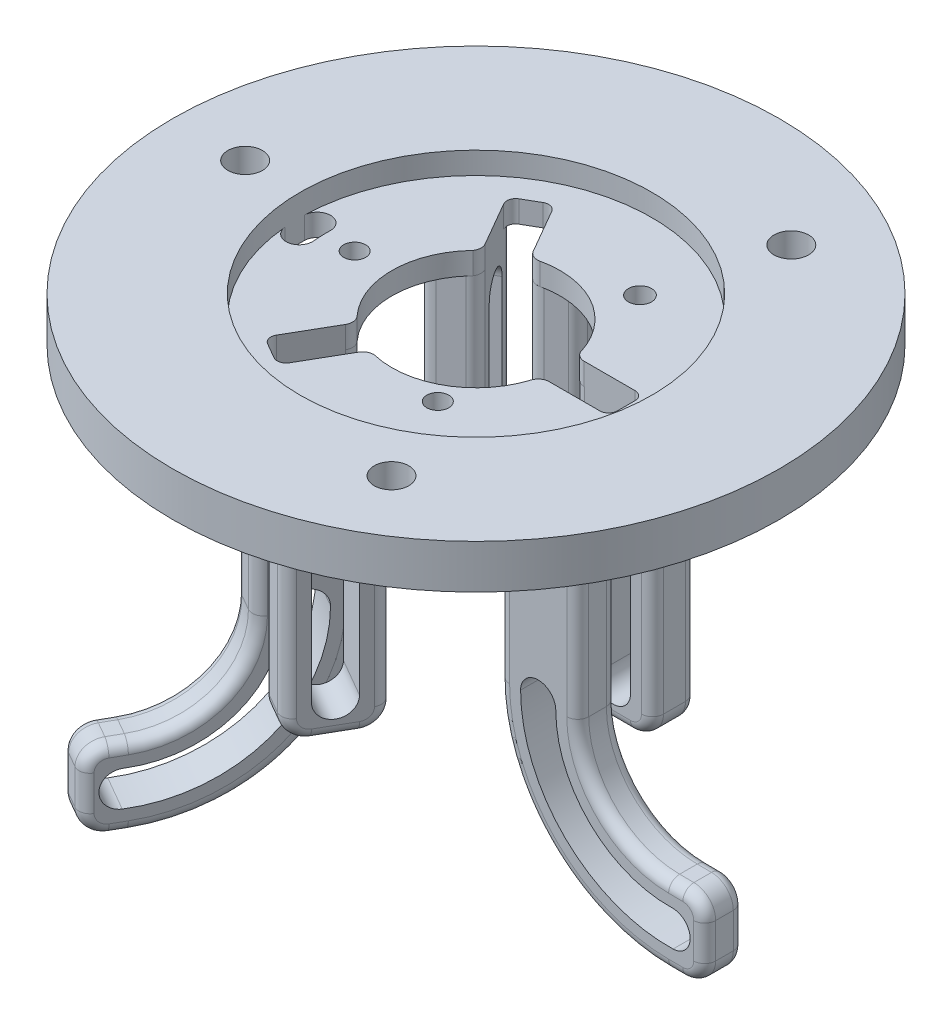
from build123d import *

# Parameters (mm, degrees)
SKETCH1_R           = 138
BOSS_EXTRUDE1_DEPTH = 20
BOSS_EXTRUDE2_START = 8
BOSS_EXTRUDE2_DEPTH = 18
CUT_EXTRUDE5_DEPTH  = 34
BOSS_EXTRUDE3_START = -70
SKETCH7_W           = 46
SKETCH7_H           = 125.96740774
BOSS_EXTRUDE3_DEPTH = 20
CUT_EXTRUDE6_START  = -72
CUT_EXTRUDE6_DEPTH  = 45
CUT_EXTRUDE7_DEPTH  = 72
CIRPATTERN1_COUNT   = 3
CUT_EXTRUDE8_DEPTH  = 27
CUT_EXTRUDE10_DEPTH = 27
CIRPATTERN4_COUNT   = 3
CIRPATTERN5_COUNT   = 3
FILLET2_R           = 10
SKETCH12_R          = 7.875
CUT_EXTRUDE11_DEPTH = 27
CIRPATTERN8_COUNT   = 3
FILLET3_R           = 5
CUT_EXTRUDE12_DEPTH = 27
CUT_EXTRUDE13_DEPTH = 27
SKETCH17_R          = 80
CUT_EXTRUDE14_DEPTH = 10
CUT_EXTRUDE15_DEPTH = 10
SKETCH19_R          = 5
SKETCH19_R_2        = 5.269356663
CUT_EXTRUDE16_DEPTH = 10


with BuildPart() as part:
    # Sketch1 → Boss-Extrude1 (new body)
    with BuildSketch(Plane(origin=(0, 0, 0), x_dir=(1, 0, 0), z_dir=(0, 1, 0))):
        with Locations(Location((0, 0, 0), (0, 0, 270))):
            Circle(SKETCH1_R)
    extrude(amount=BOSS_EXTRUDE1_DEPTH)

    # Sketch2 → Boss-Extrude2 (add)
    with BuildSketch(Plane.XY.offset(BOSS_EXTRUDE2_START)):
        Polygon((36.291327226, 0), (36.291327226, -145.182091657), (89.27461892, -189.63281459), (138, -189.63281459), (138, -149.439703236), (82.291327226, -93.731030462), (82.291327226, 0), align=None)
    boss_extrude2 = extrude(amount=BOSS_EXTRUDE2_DEPTH)

    # Sketch4 → Cut-Extrude5 (cut)
    with BuildSketch(Plane.XY.offset(8)):
        with BuildLine():
            ThreePointArc((46.291327226, -100), (66.736553538, -148.33011915), (115.658506664, -167.315645172))
            ThreePointArc((115.658506664, -167.315645172), (123.414805799, -159.07915176), (115.178312386, -151.322852625))
            ThreePointArc((115.178312386, -151.322852625), (77.879194418, -136.847891395), (62.291327226, -100))
            ThreePointArc((62.291327226, -100), (54.291327226, -92), (46.291327226, -100))
        make_face()
    cut_extrude5 = extrude(amount=CUT_EXTRUDE5_DEPTH, mode=Mode.SUBTRACT)

    # Sketch7 → Boss-Extrude3 (add)
    with BuildSketch(Plane.XY.offset(42).offset(BOSS_EXTRUDE3_START)):
        with Locations((59.291327226, -62.98370387)):
            Rectangle(SKETCH7_W, SKETCH7_H)
    boss_extrude3 = extrude(amount=BOSS_EXTRUDE3_DEPTH)

    # Sketch3 → Cut-Extrude6 (cut)
    with BuildSketch(Plane.XY.offset(26).offset(CUT_EXTRUDE6_START)):
        with BuildLine():
            Line((46.291327226, -17.246577518), (46.291327226, -110.518557102))
            ThreePointArc((46.291327226, -110.518557102), (54.291327226, -118.518557102), (62.291327226, -110.518557102))
            Line((62.291327226, -110.518557102), (62.291327226, -17.246577518))
            ThreePointArc((62.291327226, -17.246577518), (54.291327226, -9.246577518), (46.291327226, -17.246577518))
        make_face()
    cut_extrude6 = extrude(amount=CUT_EXTRUDE6_DEPTH, mode=Mode.SUBTRACT)

    # Sketch8 → Cut-Extrude7 (cut)
    with BuildSketch(Plane.XY.offset(26)):
        Polygon((138, -149.439703236), (130.041059052, -141.480762288), (130.041059052, -169.782953928), (130.057177794, -189.63281459), (138, -189.63281459), align=None)
    cut_extrude7 = extrude(amount=-CUT_EXTRUDE7_DEPTH, mode=Mode.SUBTRACT)

    # CirPattern1: Boss-Extrude2, Cut-Extrude5, Boss-Extrude3, Cut-Extrude6, Cut-Extrude7 ×3 about axis
    cirpattern1_axis = Axis((0, 0, 0), (0, 1, 0))
    add([boss_extrude2.rotate(cirpattern1_axis, i * 360 / CIRPATTERN1_COUNT) for i in range(1, CIRPATTERN1_COUNT)])
    add([cut_extrude5.rotate(cirpattern1_axis, i * 360 / CIRPATTERN1_COUNT) for i in range(1, CIRPATTERN1_COUNT)], mode=Mode.SUBTRACT)
    add([boss_extrude3.rotate(cirpattern1_axis, i * 360 / CIRPATTERN1_COUNT) for i in range(1, CIRPATTERN1_COUNT)])
    add([cut_extrude6.rotate(cirpattern1_axis, i * 360 / CIRPATTERN1_COUNT) for i in range(1, CIRPATTERN1_COUNT)], mode=Mode.SUBTRACT)
    add([cut_extrude7.rotate(cirpattern1_axis, i * 360 / CIRPATTERN1_COUNT) for i in range(1, CIRPATTERN1_COUNT)], mode=Mode.SUBTRACT)

    # Sketch9 → Cut-Extrude8 (cut)
    with BuildSketch(Plane(origin=(0, 0, -28), x_dir=(-1, 0, 0), z_dir=(0, 0, -1))):
        Polygon((-72.291327226, -43.273748779), (-72.291327226, 0), (-82.291327226, 0), (-82.291327226, -125.96740774), (-72.291327226, -125.96740774), align=None)
    cut_extrude8 = extrude(amount=-CUT_EXTRUDE8_DEPTH, mode=Mode.SUBTRACT)

    # Sketch11 → Cut-Extrude10 (cut)
    with BuildSketch(Plane.XY.offset(26)):
        with BuildLine():
            Line((36.291327226, -100), (36.291327226, -145.182091657))
            Line((36.291327226, -145.182091657), (89.27461892, -189.63281459))
            Line((89.27461892, -189.63281459), (130.057177794, -189.63281459))
            Line((130.057177794, -189.63281459), (134.49428622, -177.345982234))
            Line((134.49428622, -177.345982234), (113.63730946, -177.345982234))
            ThreePointArc((113.63730946, -177.345982234), (58.945440925, -154.691868535), (36.291327226, -100))
        make_face()
        with BuildLine():
            Line((72.28730946, -100), (72.28730946, 0))
            Line((72.28730946, 0), (138, 0))
            Line((138, 0), (154.98730946, -100))
            ThreePointArc((154.98730946, -100), (151.644308961, -116.287740448), (142.155846877, -129.941869073))
            Line((142.155846877, -129.941869073), (130.041059052, -141.480762288))
            Line((130.041059052, -141.480762288), (113.63730946, -141.35))
            ThreePointArc((113.63730946, -141.35), (84.398444058, -129.238865402), (72.28730946, -100))
        make_face()
    cut_extrude10 = extrude(amount=-CUT_EXTRUDE10_DEPTH, mode=Mode.SUBTRACT)

    # CirPattern4: Cut-Extrude8 ×3 about axis
    cirpattern4_axis = Axis((0, 20, 0), (0, -1, 0))
    for i in range(1, CIRPATTERN4_COUNT):
        add(cut_extrude8.rotate(cirpattern4_axis, i * 360 / CIRPATTERN4_COUNT), mode=Mode.SUBTRACT)

    # CirPattern5: Cut-Extrude10 ×3 about axis
    cirpattern5_axis = Axis((0, 0, 0), (0, 1, 0))
    for i in range(1, CIRPATTERN5_COUNT):
        add(cut_extrude10.rotate(cirpattern5_axis, i * 360 / CIRPATTERN5_COUNT), mode=Mode.SUBTRACT)

    # Fillet2
    fillet2_edges = [part.edges().sort_by_distance(p)[0] for p in [
        (-2.557206345, -125.96740774, 40.429211315),
        (-33.734120881, -125.96740774, -22.429211315),
        (-79.74296139, -141.480762288, 104.118860674),
        (-50.298097662, -141.480762288, -121.118860674),
        (72.291327226, -125.96740774, -18),
        (130.04720048, -177.345982234, 17),
        (-51.734120881, -125.96740774, -53.606125851),
        (-20.557206345, -125.96740774, 71.606125851),
        (-79.746032105, -177.345982234, 104.124179307),
        (-50.301168376, -177.345982234, -121.124179307),
        (36.291327226, -125.96740774, -18),
        (130.041059052, -141.480762288, 17),
    ]]
    fillet(fillet2_edges, radius=FILLET2_R)

    # Sketch12 → Cut-Extrude11 (cut)
    with BuildSketch(Plane(origin=(0, 20, 0), x_dir=(1, 0, 0), z_dir=(0, 1, 0))):
        with Locations(Location((-105, 0, 0), (0, 0, 270))):
            Circle(SKETCH12_R)
    cut_extrude11 = extrude(amount=-CUT_EXTRUDE11_DEPTH, mode=Mode.SUBTRACT)

    # CirPattern8: Cut-Extrude11 ×3 about axis
    cirpattern8_axis = Axis((0, 0, 0), (0, 1, 0))
    for i in range(1, CIRPATTERN8_COUNT):
        add(cut_extrude11.rotate(cirpattern8_axis, i * 360 / CIRPATTERN8_COUNT), mode=Mode.SUBTRACT)

    # Fillet3
    fillet3_edges = [part.edges().sort_by_distance(p)[0] for p in [
        (-25.073866843, -50, 27.429211315),
        (36.291327226, -50, 26),
        (-40.662324111, -50, 18.429211315),
        (-11.217460383, -50, -35.429211315),
        (4.370996885, -50, -44.429211315),
        (6.103047693, -57.98370387, 45.429211315),
        (-11.217460383, -57.98370387, 35.429211315),
        (-42.394374919, -57.98370387, -17.429211315),
        (-25.073866843, -57.98370387, -27.429211315),
        (72.291327226, -57.98370387, -8),
        (58.945440925, -154.691868535, 8),
        (58.945440925, -154.691868535, 26),
        (72.28730946, -50, 26),
        (84.398444058, -129.238865402, 26),
        (116.879040428, -141.375841419, 26),
        (84.398444058, -129.238865402, 8),
        (72.28730946, -50, 8),
        (116.879040428, -141.375841419, 8),
        (-43.073866843, -57.98370387, -58.606125851),
        (-29.217460383, -57.98370387, 66.606125851),
        (-22.544517232, -154.691868535, -55.048249278),
        (-6.956059964, -154.691868535, -64.048249278),
        (-58.660315228, -50, 49.602646364),
        (-64.715882527, -129.238865402, 60.091196594),
        (-80.956180712, -141.375841419, 88.220218181),
        (-49.127425259, -129.238865402, 69.091196594),
        (-43.07185796, -50, 58.602646364),
        (-65.367723444, -141.375841419, 97.220218181),
        (-36.400923693, -154.691868535, 47.048249278),
        (-51.989380961, -154.691868535, 38.048249278),
        (36.291327226, -57.98370387, -28),
        (-13.626994232, -50, -75.602646364),
        (-19.682561531, -129.238865402, -86.091196594),
        (-35.922859716, -141.375841419, -114.220218181),
        (-35.271018799, -129.238865402, -77.091196594),
        (-29.2154515, -50, -66.602646364),
        (-51.511316984, -141.375841419, -105.220218181),
        (36.291327226, -57.98370387, -8),
        (-42.503869028, -159.373673682, -125.618860674),
        (-58.092326296, -159.373673682, -116.618860674),
        (-35.90293163, -177.345982234, -114.185701723),
        (-41.039402933, -174.417050046, -123.082330993),
        (-41.053466248, -144.358536274, -123.106689369),
        (-51.491388898, -177.345982234, -105.185701723),
        (-56.627860202, -174.417050046, -114.082330993),
        (-56.641923516, -144.358536274, -114.106689369),
        (-87.537190024, -159.373673682, 99.618860674),
        (-71.948732756, -159.373673682, 108.618860674),
        (-80.936252626, -177.345982234, 88.185701723),
        (-86.07272393, -174.417050046, 97.082330993),
        (-86.086787245, -144.358536274, 97.106689369),
        (-65.347795358, -177.345982234, 97.185701723),
        (-70.484266662, -174.417050046, 106.082330993),
        (-70.498329977, -144.358536274, 106.106689369),
        (-60.394374919, -57.98370387, -48.606125851),
        (-51.394374919, -125.96740774, -33.017668583),
        (-43.858841013, -123.038475552, -19.965740996),
        (-58.929908825, -123.038475552, -46.06959617),
        (-34.073866843, -125.96740774, -43.017668583),
        (-26.538332937, -123.038475552, -29.965740996),
        (-41.609400749, -123.038475552, -56.06959617),
        (-2.896952307, -125.96740774, 61.017668583),
        (-20.217460383, -125.96740774, 51.017668583),
        (-11.896952307, -57.98370387, 76.606125851),
        (-10.432486213, -123.038475552, 74.06959617),
        (4.638581599, -123.038475552, 47.965740996),
        (-27.752994289, -123.038475552, 64.06959617),
        (-12.681926477, -123.038475552, 37.965740996),
        (54.291327226, -125.96740774, -28),
        (54.291327226, -125.96740774, -8),
        (72.291327226, -57.98370387, -28),
        (69.362395038, -123.038475552, -28),
        (39.220259414, -123.038475552, -28),
        (69.362395038, -123.038475552, -8),
        (39.220259414, -123.038475552, -8),
        (130.041059052, -159.373673682, 26),
        (130.041059052, -159.373673682, 8),
        (116.839184256, -177.345982234, 26),
        (127.112126864, -174.417050046, 26),
        (127.140253494, -144.358536274, 26),
        (116.839184256, -177.345982234, 8),
        (127.112126864, -174.417050046, 8),
        (127.140253494, -144.358536274, 8),
        (36.291327226, -50, 8),
    ]]
    fillet(fillet3_edges, radius=FILLET3_R)

    # Sketch13 → Cut-Extrude12 (cut)
    with BuildSketch(Plane.XZ):
        with BuildLine():
            Line((-39.08667554, 51.700107933), (-25.650379418, 28.427760386))
            ThreePointArc((-25.650379418, 28.427760386), (-38.289417923, 0), (-25.650379418, -28.427760386))
            Line((-25.650379418, -28.427760386), (-39.08667554, -51.700107933))
            ThreePointArc((-39.08667554, -51.700107933), (-39.48627723, -54.735384114), (-37.622573924, -57.164209549))
            Line((-37.622573924, -57.164209549), (-30.694370694, -61.164209549))
            ThreePointArc((-30.694370694, -61.164209549), (-27.659094514, -61.563811239), (-25.230269079, -59.700107933))
            Line((-25.230269079, -59.700107933), (-11.793972958, -36.427760386))
            ThreePointArc((-11.793972958, -36.427760386), (19.144708961, -33.159608617), (37.444352376, -8))
            Line((37.444352376, -8), (64.316944619, -8))
            ThreePointArc((64.316944619, -8), (67.145371743, -6.828427125), (68.316944619, -4))
            Line((68.316944619, -4), (68.316944619, 4))
            ThreePointArc((68.316944619, 4), (67.145371743, 6.828427125), (64.316944619, 8))
            Line((64.316944619, 8), (37.444352376, 8))
            ThreePointArc((37.444352376, 8), (19.144708961, 33.159608617), (-11.793972958, 36.427760386))
            Line((-11.793972958, 36.427760386), (-25.230269079, 59.700107933))
            ThreePointArc((-25.230269079, 59.700107933), (-27.659094514, 61.563811239), (-30.694370694, 61.164209549))
            Line((-30.694370694, 61.164209549), (-37.622573924, 57.164209549))
            ThreePointArc((-37.622573924, 57.164209549), (-39.48627723, 54.735384114), (-39.08667554, 51.700107933))
        make_face()
    extrude(amount=-CUT_EXTRUDE12_DEPTH, mode=Mode.SUBTRACT)

    # Sketch14 → Cut-Extrude13 (cut)
    with BuildSketch(Plane.XZ):
        with BuildLine():
            Line((-27.573866843, 31.759338334), (-13.717460383, 39.759338334))
            ThreePointArc((-13.717460383, 39.759338334), (-11.720867113, 37.810167809), (-8.994133496, 37.218074742))
            ThreePointArc((-8.994133496, 37.218074742), (18.854495266, 33.325478738), (36.534357937, 11.459503262))
            ThreePointArc((36.534357937, 11.459503262), (38.350369914, 8.956326951), (41.291327226, 8))
            Line((41.291327226, 8), (41.291327226, -8))
            ThreePointArc((41.291327226, -8), (38.6049994, -8.75451523), (36.728864955, -10.819889278))
            ThreePointArc((36.728864955, -10.819889278), (19.433463547, -32.991211245), (-8.342958029, -37.369433715))
            ThreePointArc((-8.342958029, -37.369433715), (-11.418778293, -37.690558066), (-13.717460383, -39.759338334))
            Line((-13.717460383, -39.759338334), (-27.573866843, -31.759338334))
            ThreePointArc((-27.573866843, -31.759338334), (-26.884132287, -29.055652579), (-27.734731458, -26.398185464))
            ThreePointArc((-27.734731458, -26.398185464), (-38.287958813, -0.334267493), (-28.191399908, 25.909930453))
            ThreePointArc((-28.191399908, 25.909930453), (-26.931591621, 28.734231115), (-27.573866843, 31.759338334))
        make_face()
    extrude(amount=-CUT_EXTRUDE13_DEPTH, mode=Mode.SUBTRACT)

    # Sketch17 → Cut-Extrude14 (cut)
    with BuildSketch(Plane(origin=(0, 20, 0), x_dir=(1, 0, 0), z_dir=(0, 1, 0))):
        with Locations(Location((0, 0, 0), (0, 0, 270))):
            Circle(SKETCH17_R)
    extrude(amount=-CUT_EXTRUDE14_DEPTH, mode=Mode.SUBTRACT)

    # Sketch18 → Cut-Extrude15 (cut)
    with BuildSketch(Plane(origin=(0, 10, 0), x_dir=(1, 0, 0), z_dir=(0, 1, 0))):
        with BuildLine():
            ThreePointArc((-79.976011806, 1.958962871), (-79.956460584, -2.639017031), (-79.672780672, -7.228279188))
            ThreePointArc((-79.672780672, -7.228279188), (-73.155201182, -12.661616799), (-67.721863571, -6.144037309))
            ThreePointArc((-67.721863571, -6.144037309), (-67.962991496, -2.243164477), (-67.979610036, 1.66511844))
            ThreePointArc((-67.979610036, 1.66511844), (-73.830888706, 7.810241541), (-79.976011806, 1.958962871))
        make_face()
    extrude(amount=-CUT_EXTRUDE15_DEPTH, mode=Mode.SUBTRACT)

    # Sketch19 → Cut-Extrude16 (cut)
    with BuildSketch(Plane(origin=(0, 10, 0), x_dir=(1, 0, 0), z_dir=(0, 1, 0))):
        with Locations(Location((23.75, -41.13620668, 0), (0, 0, 270))):
            Circle(SKETCH19_R)
        with Locations(Location((27.88620668, 46.6996732, 0), (0, 0, 270))):
            Circle(SKETCH19_R_2)
        with Locations(Location((-54.38620668, -0.8003268, 0), (0, 0, 270))):
            Circle(SKETCH19_R)
    extrude(amount=-CUT_EXTRUDE16_DEPTH, mode=Mode.SUBTRACT)


solid = part.part
